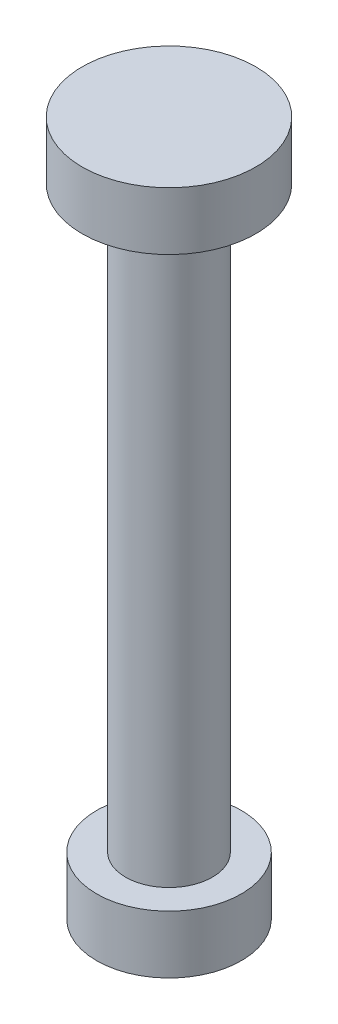
from build123d import *


with BuildPart() as part:
    # Sketch1 → Revolve1 (revolve)
    with BuildSketch(Plane.XY, mode=Mode.PRIVATE) as revolve1_sk:
        Polygon((0, 0), (2.5, 0), (2.5, 2), (1.5, 2), (1.5, 22), (3, 22), (3, 24), (0, 24), align=None)
    revolve(revolve1_sk.sketch.rotate(Axis((0, 24, 0), (0, -1, 0)), 90), axis=Axis((0, 24, 0), (0, -1, 0)))


solid = part.part
